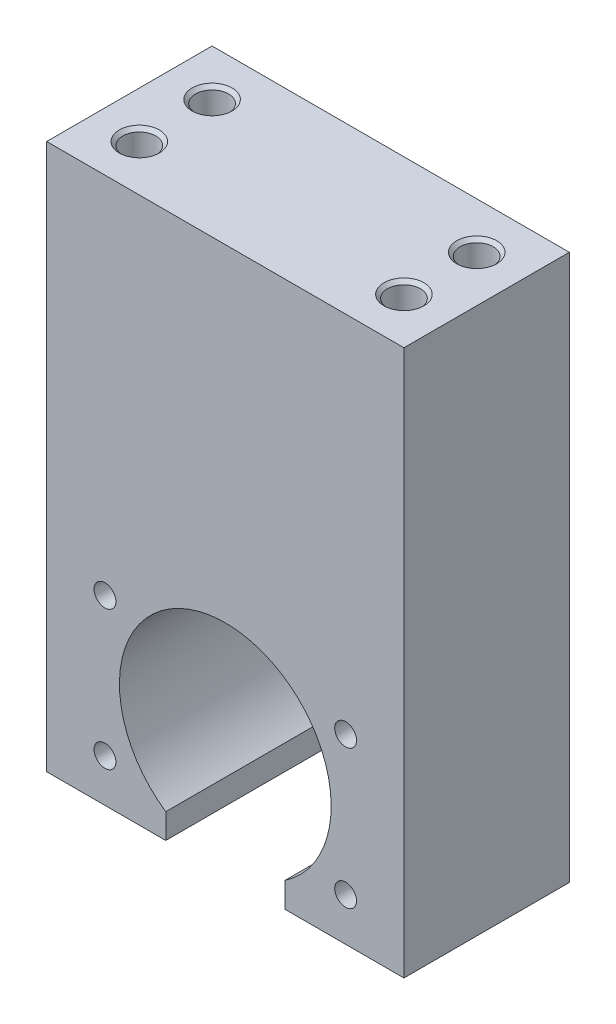
from build123d import *

# Parameters (mm, degrees)
EXTRUDE_1_DEPTH              = 12.5
HOLE_WIZARD_M4_1_D           = 3.3
HOLE_WIZARD_M4_1_DEPTH       = 9.5
HOLE_WIZARD_M4_1_TIP         = 0.991420021
HOLE_WIZARD_M6_1_D           = 5
HOLE_WIZARD_M6_1_DEPTH       = 12
HOLE_WIZARD_M6_1_CSINK_D     = 6.05
HOLE_WIZARD_M6_1_CSINK_ANGLE = 90
HOLE_WIZARD_M6_1_TIP         = 1.502151548


with BuildPart() as part:
    # 草图1 → 凸台-拉伸1 (new, symmetric)
    with BuildSketch(Plane.XY):
        with BuildLine():
            Line((-27, 65.5), (27, 65.5))
            Line((27, 65.5), (27, -17))
            Line((27, -17), (9, -17))
            Line((9, -17), (9, -13.228756555))
            ThreePointArc((9, -13.228756555), (0, 16), (-9, -13.228756555))
            Line((-9, -13.228756555), (-9, -17))
            Line((-9, -17), (-27, -17))
            Line((-27, -17), (-27, 65.5))
        make_face()
    extrude(amount=EXTRUDE_1_DEPTH, both=True)

    # M4 螺纹孔1
    with Locations(Plane.XY.offset(12.5)):
        with Locations((18.186533479, 10.5), (18.186533479, -10.5), (-18.186533479, -10.5), (-18.186533479, 10.5)):
            Hole(HOLE_WIZARD_M4_1_D / 2, depth=HOLE_WIZARD_M4_1_DEPTH)
            with Locations((0, 0, -(HOLE_WIZARD_M4_1_DEPTH + HOLE_WIZARD_M4_1_TIP / 2))):  # 118° drill point
                Cone(0, HOLE_WIZARD_M4_1_D / 2, HOLE_WIZARD_M4_1_TIP, mode=Mode.SUBTRACT)

    # M6 螺纹孔1
    with Locations(Plane(origin=(-20, 65.5, 5.5), x_dir=(0, 0, 1), z_dir=(0, 1, 0))):
        with Locations((0, 0), (-11, 0), (-11, 40), (0, 40)):
            CounterSinkHole(HOLE_WIZARD_M6_1_D / 2, HOLE_WIZARD_M6_1_CSINK_D / 2, depth=HOLE_WIZARD_M6_1_DEPTH, counter_sink_angle=HOLE_WIZARD_M6_1_CSINK_ANGLE)
            with Locations((0, 0, -(HOLE_WIZARD_M6_1_DEPTH + HOLE_WIZARD_M6_1_TIP / 2))):  # 118° drill point
                Cone(0, HOLE_WIZARD_M6_1_D / 2, HOLE_WIZARD_M6_1_TIP, mode=Mode.SUBTRACT)


solid = part.part
